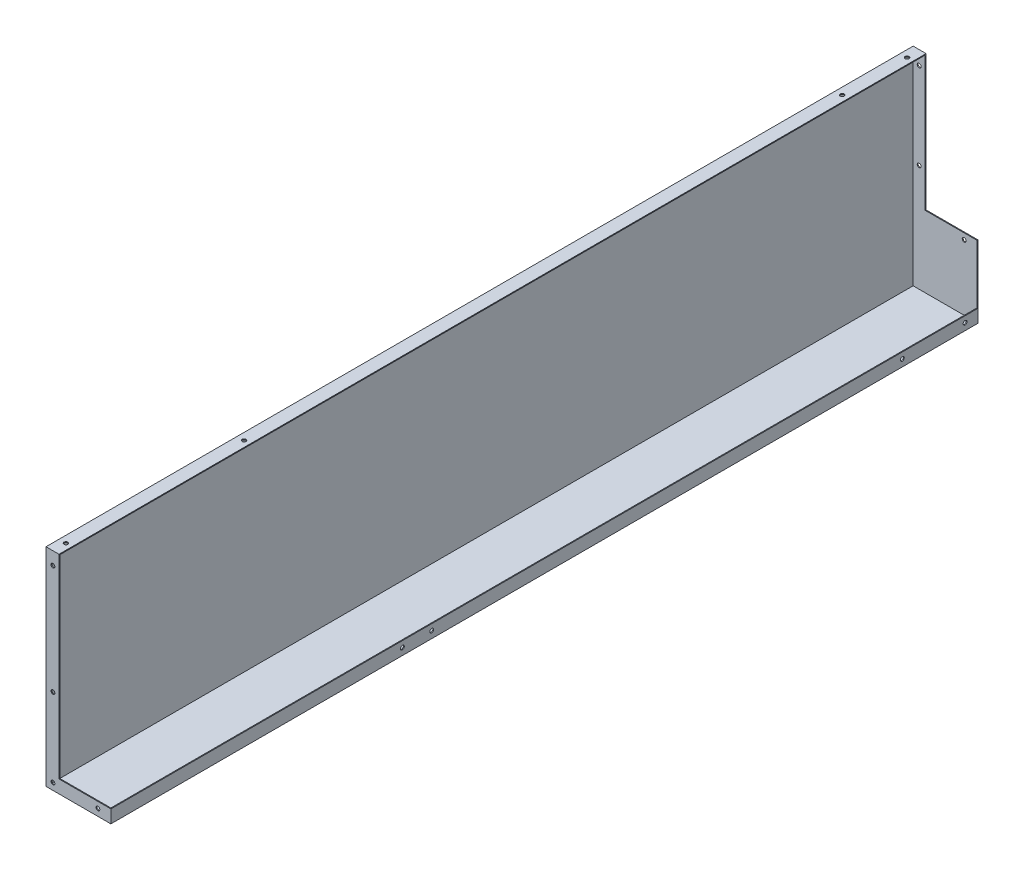
from build123d import *

# Parameters (mm, degrees)
EXTRUDE_1_DEPTH     = 2005
EXTRUDE_1_2_DEPTH   = 28
EXTRUDE_2_DEPTH     = 28
SKETCH_5_W          = 120
SKETCH_5_H          = 2
EXTRUDE_3_DEPTH     = 165
SKETCH_7_R          = 4.5
CUT_EXTRUDE_2_DEPTH = 10
SKETCH_8_R          = 4.5
CUT_EXTRUDE_3_DEPTH = 76
SKETCH_9_R          = 4.5
CUT_EXTRUDE_4_DEPTH = 10
SKETCH_10_R         = 4.5
CUT_EXTRUDE_5_DEPTH = 10
SKETCH_11_R         = 4.5
CUT_EXTRUDE_6_DEPTH = 16


with BuildPart() as part:
    # 草图1 → Extrude 1 (new body)
    with BuildSketch(Plane.XY):
        Polygon((0, 480), (0, 0), (150, 0), (150, 2), (2, 2), (2, 480), align=None)
    extrude(amount=EXTRUDE_1_DEPTH)

    # 草图3 → Extrude 1 2 (add)
    with BuildSketch(Plane(origin=(2, 0, 0), x_dir=(0, 0, -1), z_dir=(1, 0, 0))):
        Polygon((-2003, 2), (-2003, 478), (-2, 478), (-2, 2), (0, 2), (0, 480), (-2005, 480), (-2005, 2), align=None)
    extrude(amount=EXTRUDE_1_2_DEPTH)

    # 草图4 → 凸台-拉伸2 (add)
    with BuildSketch(Plane(origin=(0, 2, 0), x_dir=(1, 0, 0), z_dir=(0, 1, 0))):
        Polygon((148, -2003), (148, 0), (150, 0), (150, -2005), (30, -2005), (30, -2003), align=None)
    extrude(amount=EXTRUDE_2_DEPTH)

    # 草图5 → 凸台-拉伸3 (add)
    with BuildSketch(Plane(origin=(0, 2, 0), x_dir=(1, 0, 0), z_dir=(0, 1, 0))):
        with Locations((90, -1)):
            Rectangle(SKETCH_5_W, SKETCH_5_H)
    extrude(amount=EXTRUDE_3_DEPTH)

    # 草图7 → 切除-拉伸2 (cut)
    with BuildSketch(Plane.XY.offset(2)):
        with Locations((120, 153)):
            Circle(SKETCH_7_R)
        with Locations((16, 450)):
            Circle(SKETCH_7_R)
        with Locations((16, 250)):
            Circle(SKETCH_7_R)
    extrude(amount=-CUT_EXTRUDE_2_DEPTH, mode=Mode.SUBTRACT)

    # 草图8 → 切除-拉伸3 (cut)
    with BuildSketch(Plane.XZ.offset(-478)):
        with Locations((16, 30)):
            Circle(SKETCH_8_R)
        with Locations((16, 180)):
            Circle(SKETCH_8_R)
    extrude(amount=-CUT_EXTRUDE_3_DEPTH, mode=Mode.SUBTRACT)

    # 草图9 → 切除-拉伸4 (cut)
    with BuildSketch(Plane.XZ.offset(-478)):
        with Locations((16, 1975)):
            Circle(SKETCH_9_R)
        with Locations((16, 1563)):
            Circle(SKETCH_9_R)
    extrude(amount=-CUT_EXTRUDE_4_DEPTH, mode=Mode.SUBTRACT)

    # 草图10 → 切除-拉伸5 (cut)
    with BuildSketch(Plane.XY.offset(2005)):
        with Locations((16, 450)):
            Circle(SKETCH_10_R)
        with Locations((16, 197)):
            Circle(SKETCH_10_R)
        with Locations((16, 16)):
            Circle(SKETCH_10_R)
        with Locations((120, 16)):
            Circle(SKETCH_10_R)
    extrude(amount=-CUT_EXTRUDE_5_DEPTH, mode=Mode.SUBTRACT)

    # 草图11 → 切除-拉伸6 (cut)
    with BuildSketch(Plane(origin=(150, 0, 0), x_dir=(0, 0, -1), z_dir=(1, 0, 0))):
        with Locations((-30, 16)):
            Circle(SKETCH_11_R)
        with Locations((-175, 16)):
            Circle(SKETCH_11_R)
        with Locations((-1331, 16)):
            Circle(SKETCH_11_R)
        with Locations((-1263, 16)):
            Circle(SKETCH_11_R)
    extrude(amount=-CUT_EXTRUDE_6_DEPTH, mode=Mode.SUBTRACT)


solid = part.part
